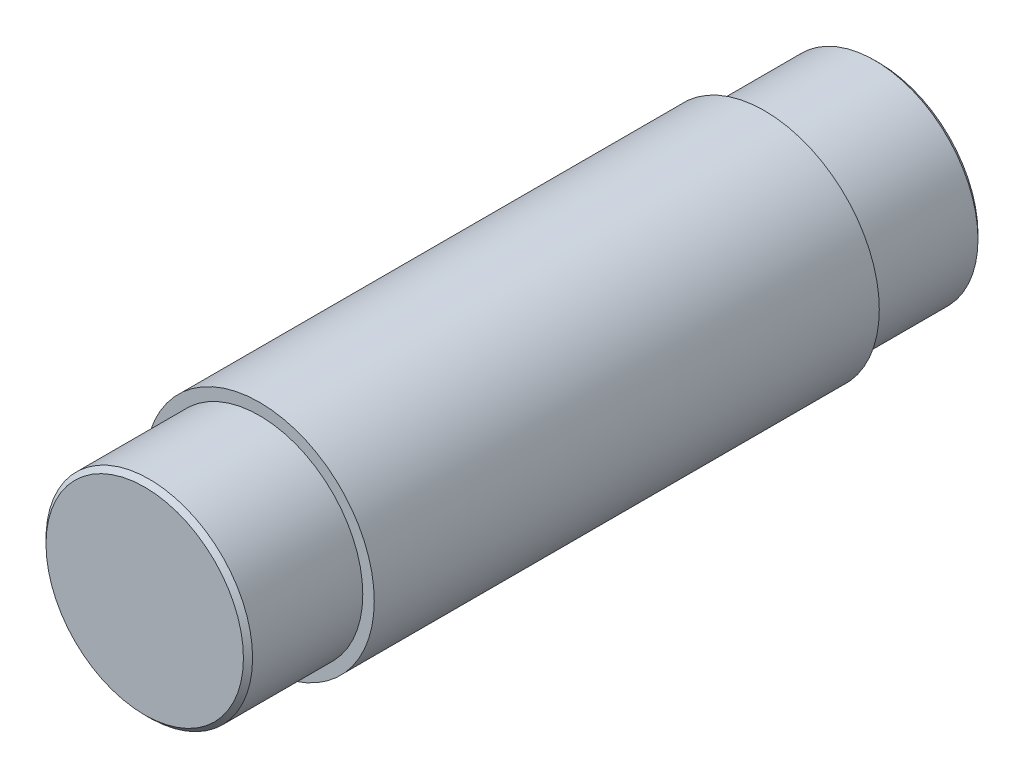
SolidWorks part; units mm, degrees
material "普通碳钢"
ref_plane "前视基准面" through (0, 0, 0) normal (0, 0, 1) x (1, 0, 0)
ref_plane "上视基准面" through (0, 0, 0) normal (0, 1, 0) x (1, 0, 0)
ref_plane "右视基准面" through (0, 0, 0) normal (1, 0, 0) x (0, 0, -1)
sketch "草图1" plane through (0, 0, 0) normal (0, 0, 1) x (1, 0, 0)
  circle A0 centre (0, 0) radius 25
  dimension "D1" = 50
extrude "凸台-拉伸1" add sketch "草图1" along normal mid plane 110
sketch "草图2" plane through (0, 0, 55) normal (0, 0, 1) x (1, 0, 0)
  circle A0 centre (0, 0) radius 22.5
  dimension "D1" = 45
extrude "凸台-拉伸2" add sketch "草图2" along normal blind 25
sketch "草图3" plane through (0, 0, -55) normal (0, 0, -1) x (-1, 0, 0)
  circle A0 centre (0, 0) radius 22.5
  dimension "D1" = 45
extrude "凸台-拉伸3" add sketch "草图3" along normal blind 25
chamfer "倒角1" distance 1 angle 45 2 edges at (22.5, 0, 80) (-22.5, 0, -80)
